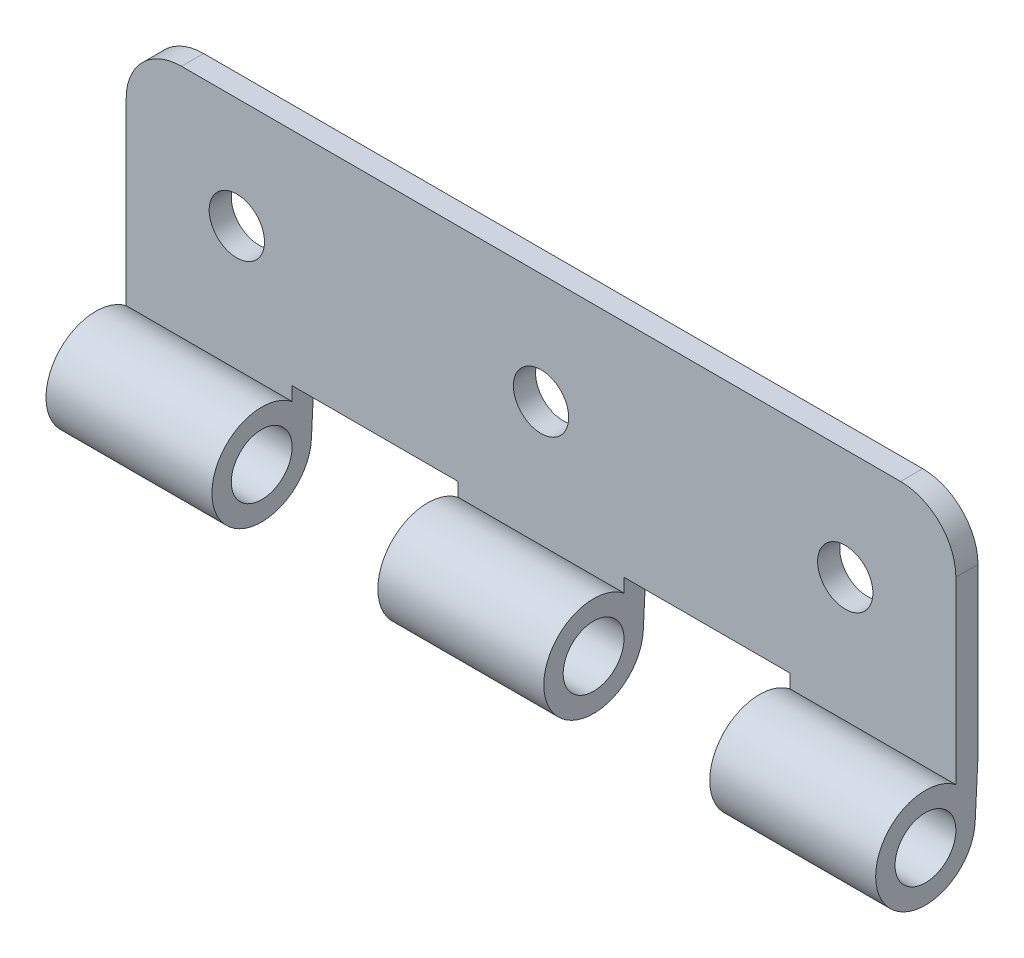
SolidWorks part; units mm, degrees
ref_plane "Front Plane" through (0, 0, 0) normal (0, 0, 1) x (1, 0, 0)
ref_plane "Top Plane" through (0, 0, 0) normal (0, 1, 0) x (1, 0, 0)
ref_plane "Right Plane" through (0, 0, 0) normal (1, 0, 0) x (0, 0, -1)
sketch "Sketch1" plane through (0, 0, 0) normal (0, 0, 1) x (1, 0, 0)
  line L0 (10, -10) -> (65, -10) construction
  line L1 (0, 0) -> (75, 0)
  line L2 (0, 0) -> (0, -20)
  line L3 (0, -20) -> (75, -20)
  line L4 (75, 0) -> (75, -20)
  line L5 (0, 0) -> (75, -20) construction
  line L6 (0, -20) -> (75, 0) construction
  circle A0 centre (10, -10) radius 2.5
  circle A1 centre (65, -10) radius 2.5
  circle A2 centre (37.5, -10) radius 2.5
  point P4 (37.5, -10)
  point P12 (37.5, -10)
  dimension "D3" = 5
  dimension "D1" = 75
  dimension "D2" = 20
  dimension "D4" = 55
extrude "Boss-Extrude1" add sketch "Sketch1" along normal blind 2
sketch "Sketch2" plane through (0, 0, 0) normal (-1, 0, 0) x (0, 0, 1)
  line L0 (2, -20) -> (2, -36.7398) construction
  line L1 (2, 0) -> (0, 0) construction
  line L3 (2, -20) -> (2, -21.238)
  line L4 (0, -20) -> (0.2558, -25.0286)
  arc A0 (0.2558, -25.0286) -> (2, -21.238) centre (4.75, -24.8) ccw
  circle A1 centre (4.75, -24.8) radius 2.75
  line M5 (0, -20) -> (2, -20)
  dimension "D1" = 9
  dimension "D2" = 5.5
  dimension "D3" = 24.8
extrude "Boss-Extrude2" add sketch "Sketch2" against normal blind 15 contours A0 L0 A1 | L0 L3 L4 A0 M5
pattern_linear "LPattern1" count 3 spacing 30 along (1, 0, 0) of "Boss-Extrude2"
fillet "Fillet1" radius 5 2 edges at (75, 0, 1) (0, 0, 1)
